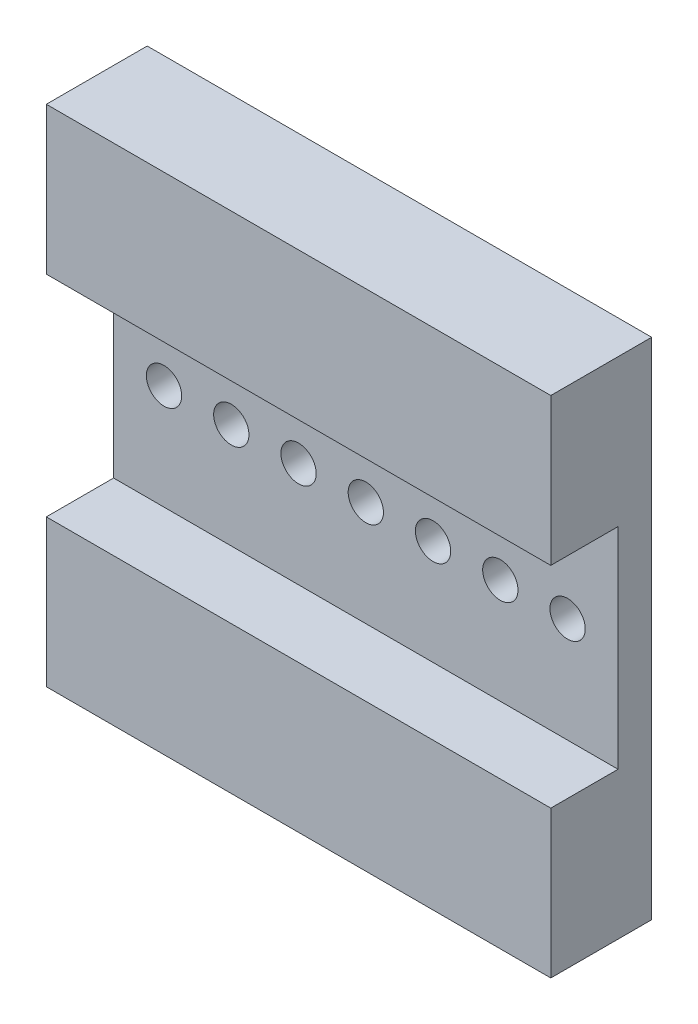
from build123d import *

# Parameters (mm, degrees)
SKETCH_1_W             = 60
SKETCH_1_H             = 60
EXTRUDE_1_DEPTH        = 12
SKETCH_2_W             = 60
SKETCH_2_H             = 25
CUT_EXTRUDE_1_DEPTH    = 8
HOLE_WIZARD_M5_1_D     = 4.2
PATTERN_LINEAR_1_COUNT = 4
PATTERN_LINEAR_1_PITCH = 8
MIRROR_1_COPY_1_D      = 4.2
MIRROR_1_COPY_2_D      = 4.2
MIRROR_1_COPY_3_D      = 4.2
MIRROR_1_COPY_4_D      = 4.2


with BuildPart() as part:
    # 草图1 → 凸台-拉伸1 (new body)
    with BuildSketch(Plane.XY):
        Rectangle(SKETCH_1_W, SKETCH_1_H)
    extrude(amount=EXTRUDE_1_DEPTH)

    # 草图2 → 切除-拉伸1 (cut)
    with BuildSketch(Plane.XY.offset(12)):
        Rectangle(SKETCH_2_W, SKETCH_2_H)
    extrude(amount=-CUT_EXTRUDE_1_DEPTH, mode=Mode.SUBTRACT)

    # M5 螺纹孔1 (through all)
    with Locations(Plane.XY.offset(4)):
        with Locations((0, 0)):
            hole_wizard_m5_1 = Hole(HOLE_WIZARD_M5_1_D / 2)

    # 阵列(线性)1: M5 螺纹孔1 ×4
    with Locations(*[(-i * PATTERN_LINEAR_1_PITCH, 0, 0) for i in range(1, PATTERN_LINEAR_1_COUNT)]):
        add(hole_wizard_m5_1, mode=Mode.SUBTRACT)

    # 镜向1 copy 1 (through all)
    with Locations(Plane(origin=(8, 0, 4), x_dir=(-1, 0, 0), z_dir=(0, 0, 1))):
        with Locations((0, 0)):
            Hole(MIRROR_1_COPY_1_D / 2)

    # 镜向1 copy 2 (through all)
    with Locations(Plane(origin=(16, 0, 4), x_dir=(-1, 0, 0), z_dir=(0, 0, 1))):
        with Locations((0, 0)):
            Hole(MIRROR_1_COPY_2_D / 2)

    # 镜向1 copy 3 (through all)
    with Locations(Plane(origin=(24, 0, 4), x_dir=(-1, 0, 0), z_dir=(0, 0, 1))):
        with Locations((0, 0)):
            Hole(MIRROR_1_COPY_3_D / 2)

    # 镜向1 copy 4 (through all)
    with Locations(Plane(origin=(0, 0, 4), x_dir=(-1, 0, 0), z_dir=(0, 0, 1))):
        with Locations((0, 0)):
            Hole(MIRROR_1_COPY_4_D / 2)


solid = part.part
